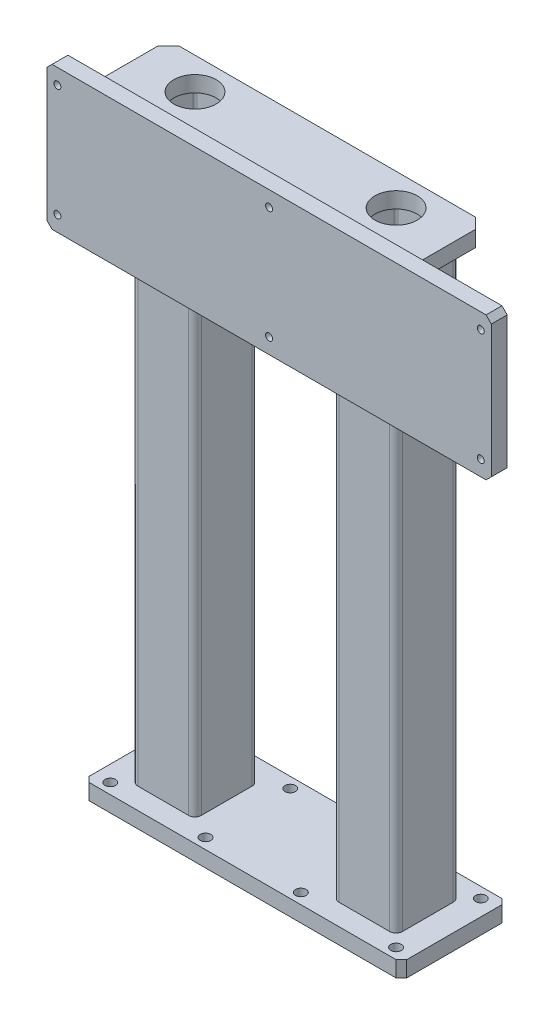
from build123d import *

# Parameters (mm, degrees)
SKETCH_1_W                  = 300
SKETCH_1_H                  = 100
EXTRUDE_1_DEPTH             = 15
EXTRUDE_2_DEPTH             = 550
SKETCH_3_W                  = 300
SKETCH_3_H                  = 100
SKETCH_3_R                  = 20
EXTRUDE_3_DEPTH             = 15
SKETCH_4_W                  = 420
SKETCH_4_H                  = 135
EXTRUDE_4_DEPTH             = 15
HOLE_WIZARD_1_AT_2_COUNT    = 2
HOLE_WIZARD_1_AT_2_PITCH    = 106
PATTERN_LINEAR_1_COUNT      = 3
PATTERN_LINEAR_1_PITCH      = 200
SKETCH_7_R                  = 20
CUT_EXTRUDE_1_DEPTH         = 668.944608482
CHAMFER_1_SIZE              = 10
CHAMFER_2_SIZE              = 5
EXTRUDE_5_REACH             = 688.804
SKETCH_8_W                  = 15
SKETCH_8_H                  = 80
SKETCH_9_R                  = 5
CUT_EXTRUDE_2_DEPTH         = 668.944608482
PATTERN_LINEAR_2_COUNT      = 4
PATTERN_LINEAR_2_PITCH      = 90
PATTERN_LINEAR_2_COUNT_DIR2 = 2
PATTERN_LINEAR_2_PITCH_DIR2 = 80
CHAMFER_3_SIZE              = 5
CUT_EXTRUDE_3_DEPTH         = 5


with BuildPart() as part:
    # 草图1 → 凸台-拉伸1 (new body)
    with BuildSketch(Plane(origin=(0, 0, 0), x_dir=(1, 0, 0), z_dir=(0, 1, 0))):
        Rectangle(SKETCH_1_W, SKETCH_1_H)
    extrude(amount=EXTRUDE_1_DEPTH)

    # 草图2 → 凸台-拉伸2 (add)
    # profile 1 of 2: a face of its own
    with BuildSketch(Plane(origin=(0, 15, 0), x_dir=(1, 0, 0), z_dir=(0, 1, 0))):
        with BuildLine():
            Line((-119, 30), (-71, 30))
            ThreePointArc((-71, 30), (-66.757359313, 28.242640687), (-65, 24))
            Line((-65, 24), (-65, -24))
            ThreePointArc((-65, -24), (-66.757359313, -28.242640687), (-71, -30))
            Line((-71, -30), (-119, -30))
            ThreePointArc((-119, -30), (-123.242640687, -28.242640687), (-125, -24))
            Line((-125, -24), (-125, 24))
            ThreePointArc((-125, 24), (-123.242640687, 28.242640687), (-119, 30))
        make_face()
        with BuildLine():
            Line((-119, 26), (-71, 26))
            ThreePointArc((-71, 26), (-69.585786438, 25.414213562), (-69, 24))
            Line((-69, 24), (-69, -24))
            ThreePointArc((-69, -24), (-69.585786438, -25.414213562), (-71, -26))
            Line((-71, -26), (-119, -26))
            ThreePointArc((-119, -26), (-120.414213562, -25.414213562), (-121, -24))
            Line((-121, -24), (-121, 24))
            ThreePointArc((-121, 24), (-120.414213562, 25.414213562), (-119, 26))
        make_face(mode=Mode.SUBTRACT)
    # profile 2 of 2: a face of its own
    with BuildSketch(Plane(origin=(0, 15, 0), x_dir=(1, 0, 0), z_dir=(0, 1, 0))):
        with BuildLine():
            Line((65, 24), (65, -24))
            ThreePointArc((65, -24), (66.757359313, -28.242640687), (71, -30))
            Line((71, -30), (119, -30))
            ThreePointArc((119, -30), (123.242640687, -28.242640687), (125, -24))
            Line((125, -24), (125, 24))
            ThreePointArc((125, 24), (123.242640687, 28.242640687), (119, 30))
            Line((119, 30), (71, 30))
            ThreePointArc((71, 30), (66.757359313, 28.242640687), (65, 24))
        make_face()
        with BuildLine():
            Line((121, 24), (121, -24))
            ThreePointArc((121, -24), (120.414213562, -25.414213562), (119, -26))
            Line((119, -26), (71, -26))
            ThreePointArc((71, -26), (69.585786438, -25.414213562), (69, -24))
            Line((69, -24), (69, 24))
            ThreePointArc((69, 24), (69.585786438, 25.414213562), (71, 26))
            Line((71, 26), (119, 26))
            ThreePointArc((119, 26), (120.414213562, 25.414213562), (121, 24))
        make_face(mode=Mode.SUBTRACT)
    extrude(amount=EXTRUDE_2_DEPTH)

    # 草图3 → 凸台-拉伸3 (add)
    with BuildSketch(Plane(origin=(0, 565, 0), x_dir=(1, 0, 0), z_dir=(0, 1, 0))):
        with Locations((0, -20)):
            Rectangle(SKETCH_3_W, SKETCH_3_H)
        with Locations(Location((-95, 0, 0), (0, 0, 270))):
            Circle(SKETCH_3_R, mode=Mode.SUBTRACT)
        with Locations(Location((95, 0, 0), (0, 0, 270))):
            Circle(SKETCH_3_R, mode=Mode.SUBTRACT)
    extrude(amount=EXTRUDE_3_DEPTH)

    # 草图4 → 凸台-拉伸4 (add)
    with BuildSketch(Plane.XY.offset(70)):
        with Locations((60, 552.5)):
            Rectangle(SKETCH_4_W, SKETCH_4_H)
    extrude(amount=EXTRUDE_4_DEPTH)

    # 草图5 → 打孔尺寸(%根据)内六角圆柱头螺钉的类型1 (revolve, cut)
    with BuildSketch(Plane(origin=(-140, 605.5, 70), x_dir=(0, 1, 0), z_dir=(1, 0, 0))):
        Polygon((0, 0), (0, 16.982840043), (3.3, 15), (3.3, 6.8), (5.5, 6.8), (5.5, 0), align=None)
    hole_wizard_1 = revolve(axis=Axis((-140, 605.5, 63.65), (0, 0, 1)), mode=Mode.SUBTRACT)

    # 打孔尺寸(%根据)内六角圆柱头螺钉的类型1 at 2: 打孔尺寸(%根据)内六角圆柱头螺钉的类型1 ×2
    with Locations(*[(0, -i * HOLE_WIZARD_1_AT_2_PITCH, 0) for i in range(1, HOLE_WIZARD_1_AT_2_COUNT)]):
        add(hole_wizard_1, mode=Mode.SUBTRACT)

    # 阵列(线性)1: 打孔尺寸(%根据)内六角圆柱头螺钉的类型1 ×3
    with Locations(*[(i * PATTERN_LINEAR_1_PITCH, 0, 0) for i in range(1, PATTERN_LINEAR_1_COUNT)]):
        add(hole_wizard_1, mode=Mode.SUBTRACT)

    # 阵列(线性)1 copy 1 sketch → 阵列(线性)1 copy 1 (revolve, cut)
    with BuildSketch(Plane(origin=(60, 499.5, 70), x_dir=(0, 1, 0), z_dir=(1, 0, 0))):
        Polygon((0, 0), (0, 16.982840043), (3.3, 15), (3.3, 6.8), (5.5, 6.8), (5.5, 0), align=None)
    revolve(axis=Axis((60, 499.5, 63.65), (0, 0, 1)), mode=Mode.SUBTRACT)

    # 阵列(线性)1 copy 2 sketch → 阵列(线性)1 copy 2 (revolve, cut)
    with BuildSketch(Plane(origin=(260, 499.5, 70), x_dir=(0, 1, 0), z_dir=(1, 0, 0))):
        Polygon((0, 0), (0, 16.982840043), (3.3, 15), (3.3, 6.8), (5.5, 6.8), (5.5, 0), align=None)
    revolve(axis=Axis((260, 499.5, 63.65), (0, 0, 1)), mode=Mode.SUBTRACT)

    # 草图7 → 切除-拉伸1 (cut, through all)
    with BuildSketch(Plane(origin=(0, 15, 0), x_dir=(1, 0, 0), z_dir=(0, 1, 0))):
        with Locations(Location((-95, 0, 0), (0, 0, 270))):
            Circle(SKETCH_7_R)
        with Locations(Location((95, 0, 0), (0, 0, 270))):
            Circle(SKETCH_7_R)
    extrude(amount=-CUT_EXTRUDE_1_DEPTH, mode=Mode.SUBTRACT)

    # 倒角1
    chamfer_1_edges = [part.edges().sort_by_distance(p)[0] for p in [
        (-150, 572.5, -30),
        (150, 572.5, -30),
    ]]
    chamfer(chamfer_1_edges, length=CHAMFER_1_SIZE)

    # 倒角2
    chamfer_2_edges = [part.edges().sort_by_distance(p)[0] for p in [
        (270, 485, 77.5),
        (270, 620, 77.5),
        (-150, 485, 77.5),
        (-150, 620, 77.5),
    ]]
    chamfer(chamfer_2_edges, length=CHAMFER_2_SIZE)

    # 草图8 → 凸台-拉伸5 (add, up to next)
    with BuildSketch(Plane(origin=(0, 0, 70), x_dir=(-1, 0, 0), z_dir=(0, 0, -1)), mode=Mode.PRIVATE) as extrude_5_sk1:
        with Locations((-95, 525)):
            Rectangle(SKETCH_8_W, SKETCH_8_H)
    extrude_5_tool1 = extrude(extrude_5_sk1.sketch, amount=EXTRUDE_5_REACH, mode=Mode.PRIVATE) - part.part
    # 草图8 → 凸台-拉伸5 (add, up to next)
    with BuildSketch(Plane(origin=(0, 0, 70), x_dir=(-1, 0, 0), z_dir=(0, 0, -1)), mode=Mode.PRIVATE) as extrude_5_sk2:
        with Locations((95, 525)):
            Rectangle(SKETCH_8_W, SKETCH_8_H)
    extrude_5_tool2 = extrude(extrude_5_sk2.sketch, amount=EXTRUDE_5_REACH, mode=Mode.PRIVATE) - part.part
    add(extrude_5_tool1.solids().sort_by_distance((95, 525, 70))[0])
    add(extrude_5_tool2.solids().sort_by_distance((-95, 525, 70))[0])

    # 草图9 → 切除-拉伸2 (cut, through all)
    with BuildSketch(Plane(origin=(0, 15, 0), x_dir=(1, 0, 0), z_dir=(0, 1, 0))):
        with Locations(Location((-135, 40, 0), (0, 0, 270))):
            Circle(SKETCH_9_R)
    cut_extrude_2 = extrude(amount=-CUT_EXTRUDE_2_DEPTH, mode=Mode.SUBTRACT)

    # 阵列(线性)2: Cut-Extrude 2 4 × 2
    with Locations(*[(i * PATTERN_LINEAR_2_PITCH, 0, j * PATTERN_LINEAR_2_PITCH_DIR2) for i in range(PATTERN_LINEAR_2_COUNT) for j in range(PATTERN_LINEAR_2_COUNT_DIR2) if (i, j) != (0, 0)]):
        add(cut_extrude_2, mode=Mode.SUBTRACT)

    # 倒角3
    chamfer_3_edges = [part.edges().sort_by_distance(p)[0] for p in [
        (150, 7.5, 50),
        (-150, 7.5, 50),
        (-150, 7.5, -50),
        (150, 7.5, -50),
    ]]
    chamfer(chamfer_3_edges, length=CHAMFER_3_SIZE)

    # 草图10 → 切除-拉伸3 (cut)
    with BuildSketch(Plane(origin=(0, 0, -30), x_dir=(-1, 0, 0), z_dir=(0, 0, -1))):
        with BuildLine():
            Line((-107.5, 50), (-82.5, 50))
            ThreePointArc((-82.5, 50), (-78.964466094, 51.464466094), (-77.5, 55))
            Line((-77.5, 55), (-77.5, 95))
            ThreePointArc((-77.5, 95), (-78.964466094, 98.535533906), (-82.5, 100))
            Line((-82.5, 100), (-107.5, 100))
            ThreePointArc((-107.5, 100), (-111.035533906, 98.535533906), (-112.5, 95))
            Line((-112.5, 95), (-112.5, 55))
            ThreePointArc((-112.5, 55), (-111.035533906, 51.464466094), (-107.5, 50))
        make_face()
        with BuildLine():
            Line((82.5, 50), (107.5, 50))
            ThreePointArc((107.5, 50), (111.035533906, 51.464466094), (112.5, 55))
            Line((112.5, 55), (112.5, 95))
            ThreePointArc((112.5, 95), (111.035533906, 98.535533906), (107.5, 100))
            Line((107.5, 100), (82.5, 100))
            ThreePointArc((82.5, 100), (78.964466094, 98.535533906), (77.5, 95))
            Line((77.5, 95), (77.5, 55))
            ThreePointArc((77.5, 55), (78.964466094, 51.464466094), (82.5, 50))
        make_face()
    extrude(amount=-CUT_EXTRUDE_3_DEPTH, mode=Mode.SUBTRACT)


solid = part.part
